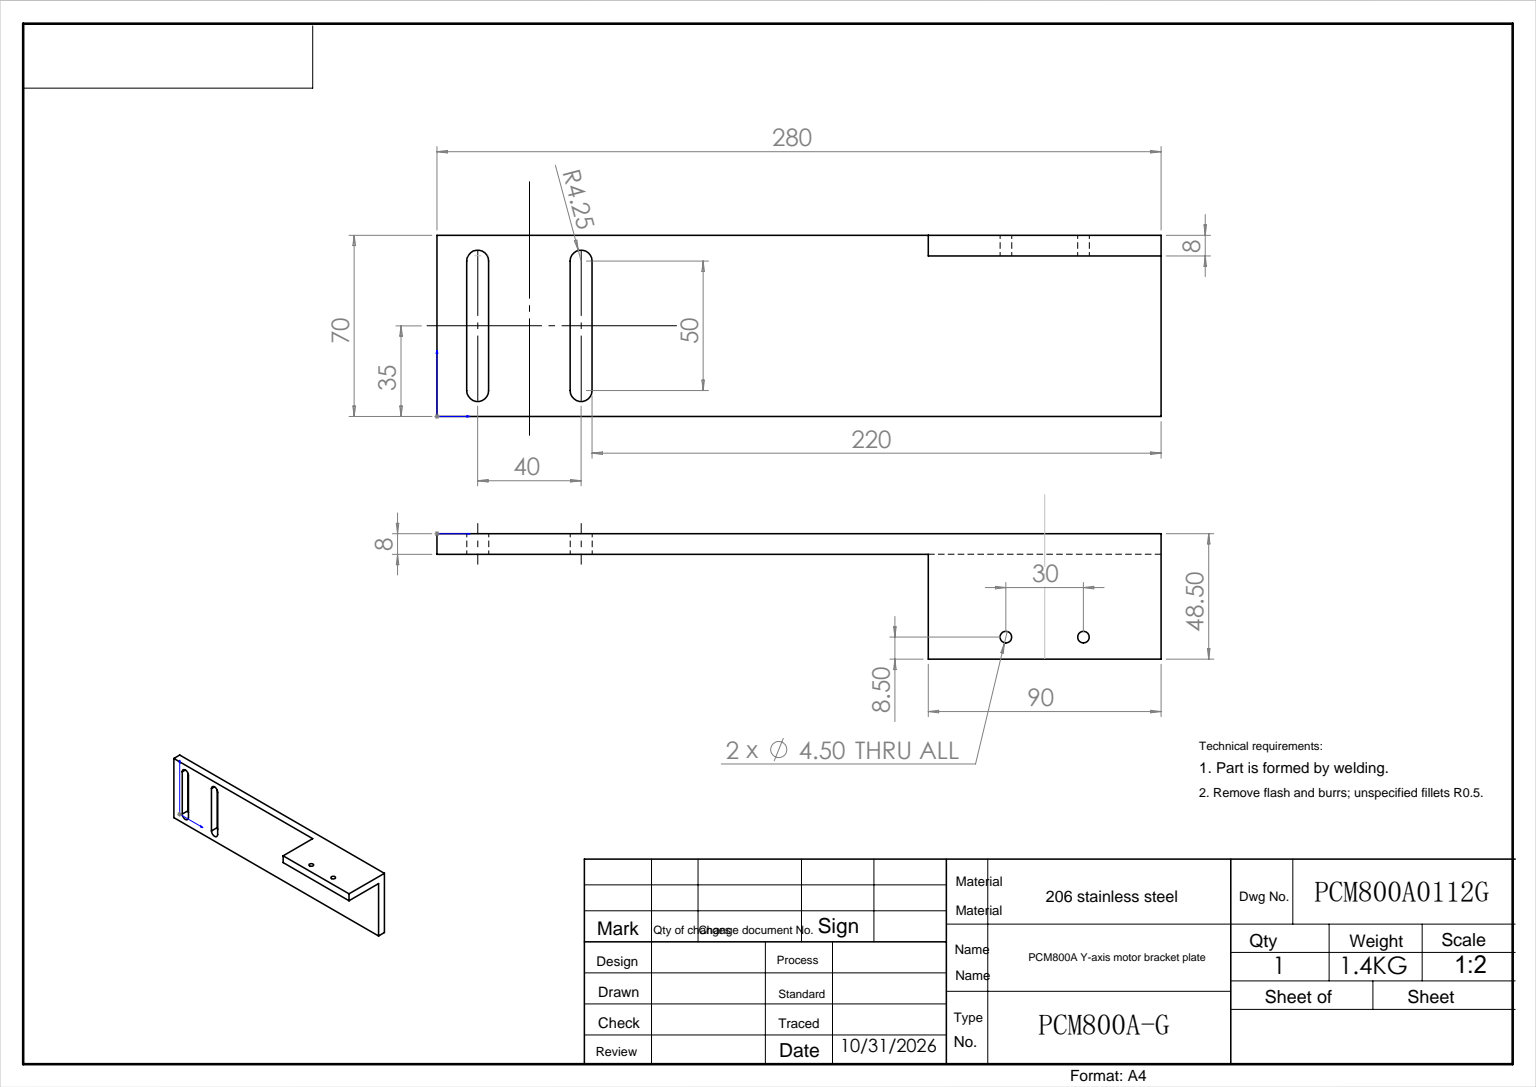
SolidWorks part; units mm, degrees
ref_plane "前视基准面" through (0, 0, 0) normal (0, 0, 1) x (1, 0, 0)
ref_plane "上视基准面" through (0, 0, 0) normal (0, 1, 0) x (1, 0, 0)
ref_plane "右视基准面" through (0, 0, 0) normal (1, 0, 0) x (0, 0, -1)
sketch "草图1" plane through (0, 0, 0) normal (0, 0, 1) x (1, 0, 0)
  line L0 (35.75, 90.0371) -> (35.75, -23.041) construction
  line L1 (0, 0) -> (280, 0)
  line L2 (0, 0) -> (0, 70)
  line L3 (0, 70) -> (280, 70)
  line L4 (280, 0) -> (280, 70)
  line L5 (0, 35) -> (256.1339, 35) construction
  line L6 (51.5, 60) -> (51.5, 10)
  line L7 (60, 60) -> (60, 10)
  line L8 (11.5, 60) -> (11.5, 10)
  line L9 (20, 60) -> (20, 10)
  arc A0 (60, 60) -> (51.5, 60) centre (55.75, 60) ccw
  arc A1 (20, 10) -> (11.5, 10) centre (15.75, 10) cw
  arc A2 (51.5, 10) -> (60, 10) centre (55.75, 10) ccw
  arc A3 (11.5, 60) -> (20, 60) centre (15.75, 60) cw
  dimension "D5" = 8.5
  dimension "D7" = 50
  dimension "D3" = 220
  dimension "D4" = 20
  dimension "D1" = 280
  dimension "D2" = 70
  dimension "D8" = 25
extrude "凸台-拉伸1" add sketch "草图1" along normal blind 8
sketch "草图2" plane through (0, 0, 8) normal (0, 0, 1) x (1, 0, 0)
  line L1 (280, 70) -> (190, 70)
  line L2 (280, 70) -> (280, 62)
  line L3 (280, 62) -> (190, 62)
  line L4 (190, 70) -> (190, 62)
  dimension "D1" = 8
  dimension "D2" = 90
extrude "凸台-拉伸2" add sketch "草图2" along normal blind 40.5
hole_wizard "Ø4.5 (4.5) 直径孔1" positions "草图4" profile "草图3" hole size "Ø4.5" standard "GB" end condition through all
sketch "草图4" plane through (0, 70, 0) normal (0, 1, 0) x (-1, 0, 0)
  line L0 (-290.8006, 40) -> (-177.6179, 40) construction
  line L2 (-280, 48.5) -> (-190, 48.5) construction
  line L3 (-235, 48.5) -> (-235, 26.5832) construction
  point P0 (-220, 40)
  point P1 (-250, 40)
  dimension "D1" = 8.5
  dimension "D2" = 15
  dimension "D3" = 30
sketch "草图3" plane through (220, 70, 40) normal (1, 0, 0) x (0, 0, 1)
  line L0 (0, 0) -> (0, 70)
  line L1 (0, 70) -> (2.25, 70)
  line L2 (2.25, 70) -> (2.25, 0)
  line L5 (2.25, 0) -> (0, 0)
  line L11 (0, -6.35) -> (0, 107.95) construction
  dimension "通孔孔直径" = 4.5
  dimension "通孔孔深度" = 70
